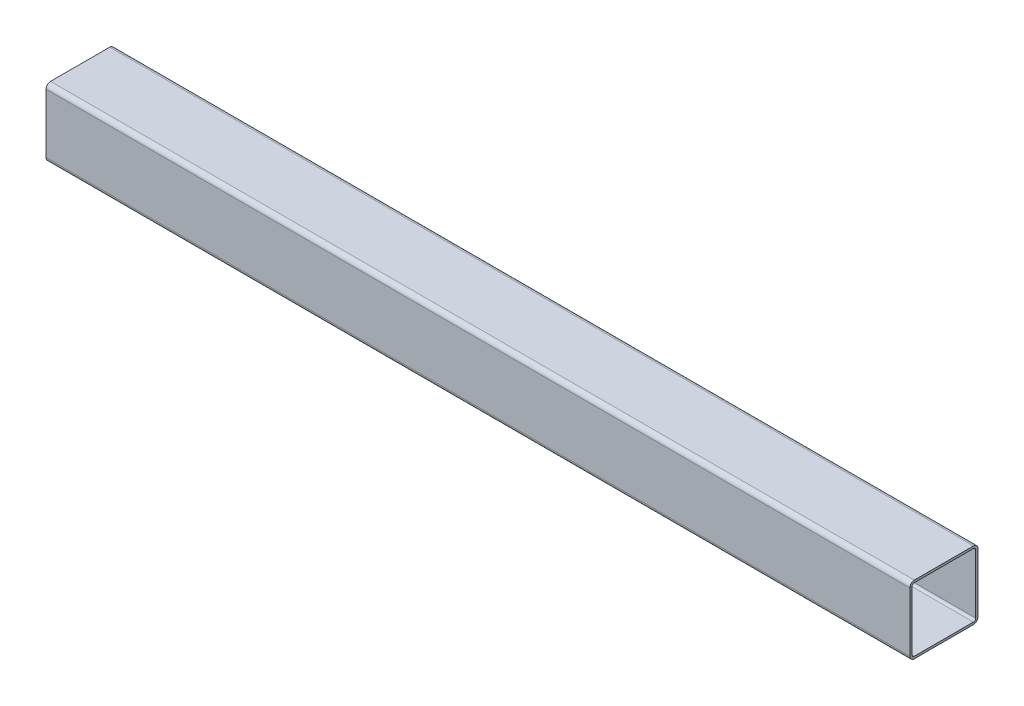
SolidWorks part; units mm, degrees
ref_plane "前视基准面" through (0, 0, 0) normal (0, 0, 1) x (1, 0, 0)
ref_plane "上视基准面" through (0, 0, 0) normal (0, 1, 0) x (1, 0, 0)
ref_plane "右视基准面" through (0, 0, 0) normal (1, 0, 0) x (0, 0, -1)
sketch "草图1" plane through (0, 0, 0) normal (0, 0, 1) x (1, 0, 0)
  line L0 (-950, 0) -> (950, 0)
  point P4 (0, 0)
  dimension "D1" = 1900
other "Gb／6728-1986方形空心型钢 150 X 150 X 5(1)"
ref_plane "基准面1" through (-950, 0, 0) normal (1, 0, 0) x (0, 1, 0)
sketch "Sketch1" plane through (-950, 0, 0) normal (1, 0, 0) x (0, 1, 0)
  line L0 (-65, -70) -> (65, -70)
  line L1 (-70, -65) -> (-70, 65)
  line L2 (65, 70) -> (-65, 70)
  line L3 (70, 65) -> (70, -65)
  line L4 (-65, -75) -> (65, -75)
  line L5 (-75, -65) -> (-75, 65)
  line L6 (65, 75) -> (-65, 75)
  line L7 (75, 65) -> (75, -65)
  arc A0 (75, 65) -> (65, 75) centre (65, 65) ccw
  arc A1 (65, -75) -> (75, -65) centre (65, -65) ccw
  arc A2 (-75, -65) -> (-65, -75) centre (-65, -65) ccw
  arc A3 (-65, 75) -> (-75, 65) centre (-65, 65) ccw
  arc A4 (-65, 70) -> (-70, 65) centre (-65, 65) ccw
  arc A5 (70, 65) -> (65, 70) centre (65, 65) ccw
  arc A6 (65, -70) -> (70, -65) centre (65, -65) ccw
  arc A7 (-70, -65) -> (-65, -70) centre (-65, -65) ccw
  point P0 (-75, 0)
  point P1 (75, 0)
  point P2 (0, 75)
  point P3 (0, -75)
  point P4 (0, 0)
  point P5 (-75, -75)
  point P6 (75, -75)
  point P7 (75, 75)
  point P8 (-75, 75)
  point P33 (0, 0)
  dimension "D1" = 10
  dimension "Thickness" = 5
  dimension "V_leg" = 150
